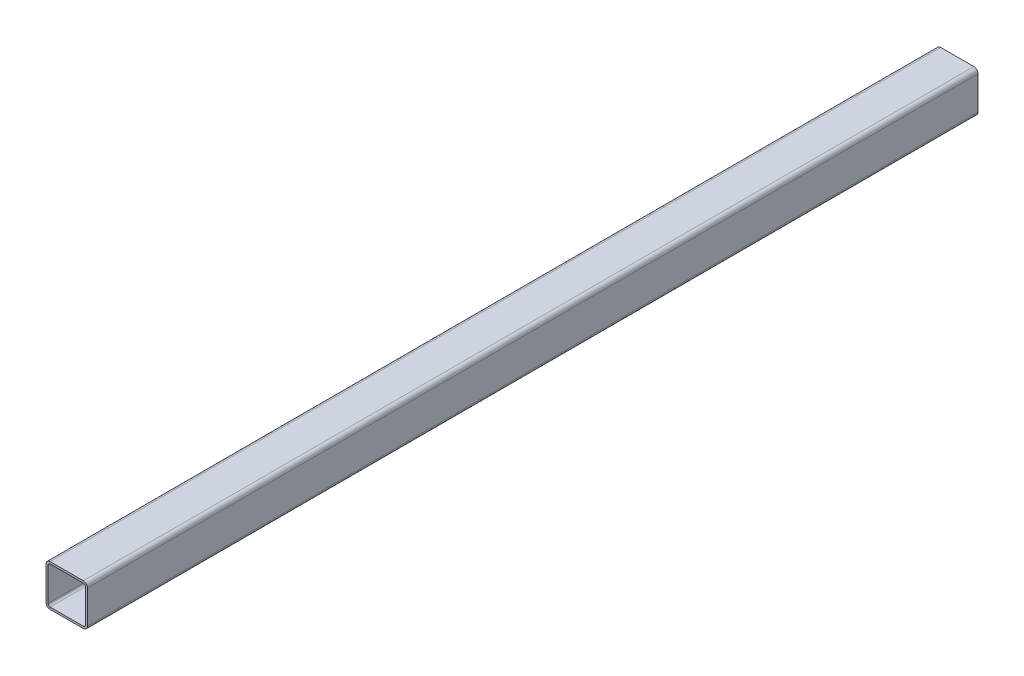
from build123d import *

# Parameters (mm, degrees)
SKETCH1_W           = 40
SKETCH1_H           = 40
SKETCH1_W_2         = 36
SKETCH1_H_2         = 36
BOSS_EXTRUDE1_DEPTH = 860
FILLET1_R           = 2
FILLET2_R           = 4


with BuildPart() as part:
    # Sketch1 → Boss-Extrude1 (new body)
    with BuildSketch(Plane.XY):
        Rectangle(SKETCH1_W, SKETCH1_H)
        Rectangle(SKETCH1_W_2, SKETCH1_H_2, mode=Mode.SUBTRACT)
    extrude(amount=BOSS_EXTRUDE1_DEPTH)

    # Fillet1
    fillet1_edges = [part.edges().sort_by_distance(p)[0] for p in [
        (18, -18, 430),
        (18, 18, 430),
        (-18, 18, 430),
        (-18, -18, 430),
    ]]
    fillet(fillet1_edges, radius=FILLET1_R)

    # Fillet2
    fillet2_edges = [part.edges().sort_by_distance(p)[0] for p in [
        (20, -20, 430),
        (-20, -20, 430),
        (-20, 20, 430),
        (20, 20, 430),
    ]]
    fillet(fillet2_edges, radius=FILLET2_R)


solid = part.part
